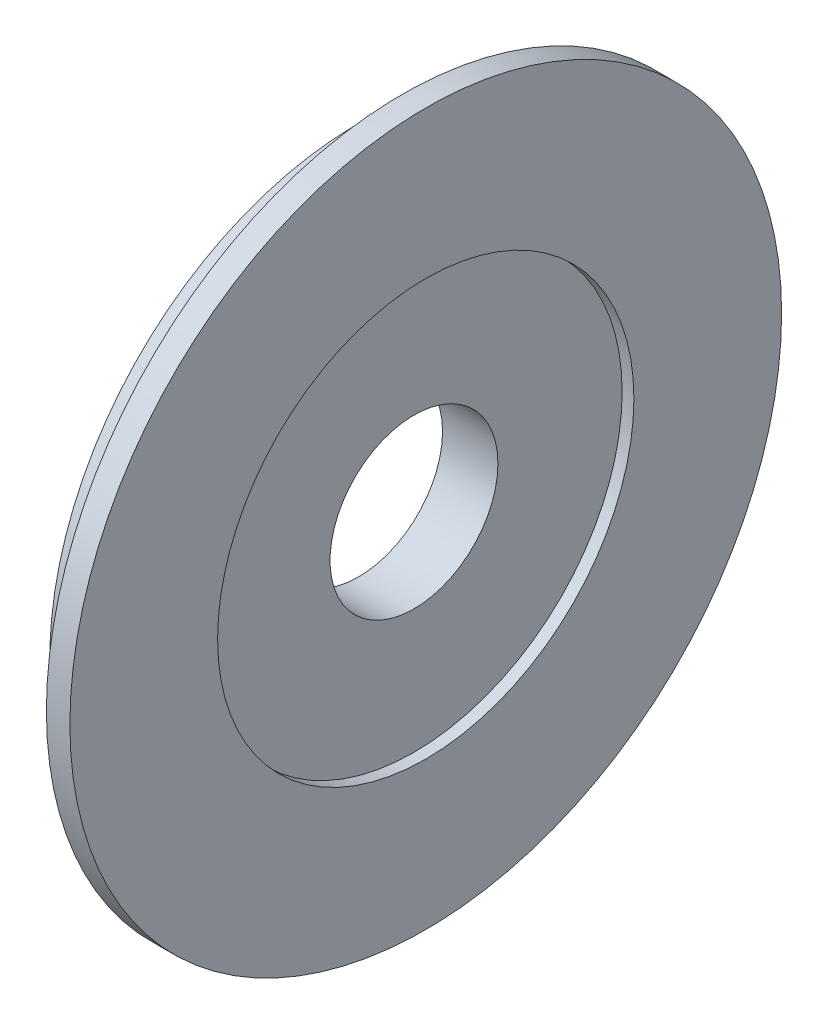
from build123d import *


with BuildPart() as part:
    # Sketch1 → Revolve1 (revolve)
    with BuildSketch(Plane.XY, mode=Mode.PRIVATE) as revolve1_sk:
        Polygon((-11.770833333, 46), (-11.770833333, 12.5), (-3.520833333, 12.5), (-3.520833333, 31), (-1.770833333, 31), (-1.770833333, 53), (-5.270833333, 53), (-7.770833333, 46), align=None)
    revolve(revolve1_sk.sketch.rotate(Axis((0, 0, 0), (-1, 0, 0)), 90), axis=Axis((0, 0, 0), (-1, 0, 0)))


solid = part.part
